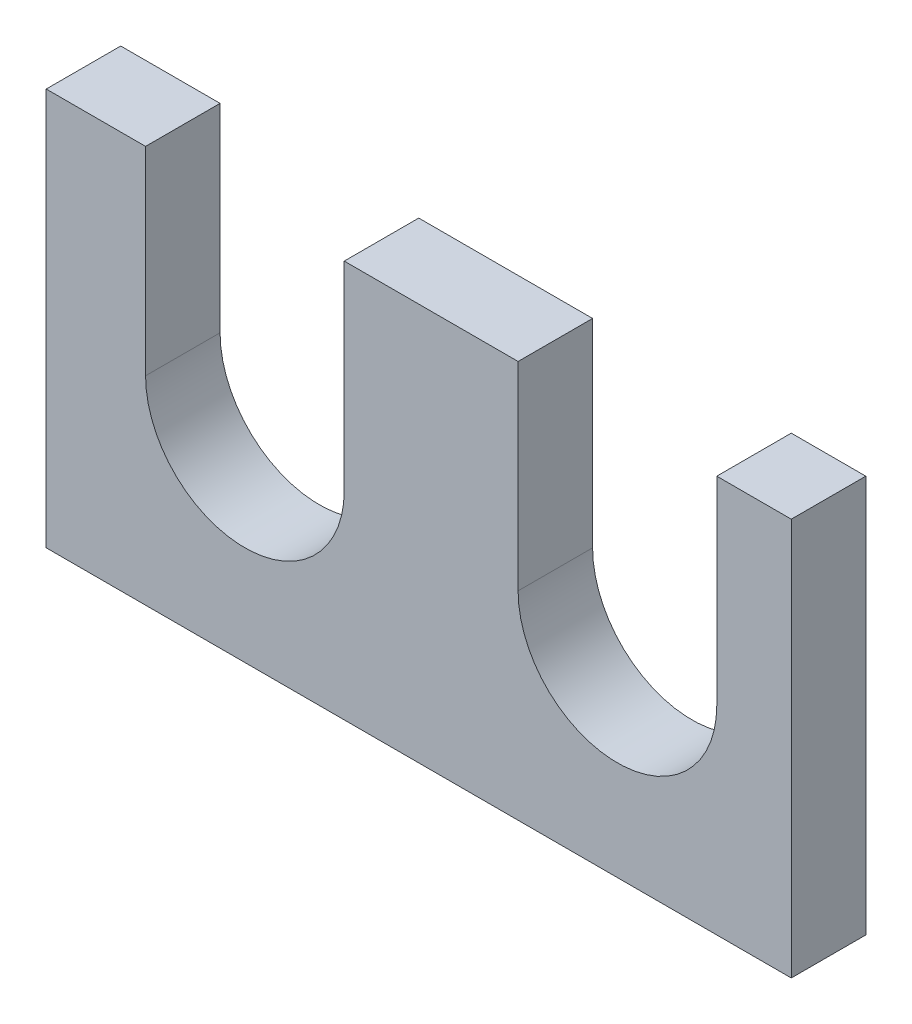
from build123d import *

# Parameters (mm, degrees)
BOSS_EXTRUDE1_DEPTH = 3


with BuildPart() as part:
    # Sketch1 → Boss-Extrude1 (new body)
    with BuildSketch(Plane.XY):
        with BuildLine():
            Line((0, 0), (30, 0))
            Line((30, 0), (30, 16))
            Line((30, 16), (27, 16))
            Line((27, 16), (27, 8))
            ThreePointArc((27, 8), (23, 4), (19, 8))
            Line((19, 8), (19, 16))
            Line((19, 16), (12, 16))
            Line((12, 16), (12, 8))
            ThreePointArc((12, 8), (8, 4), (4, 8))
            Line((4, 8), (4, 16))
            Line((4, 16), (0, 16))
            Line((0, 16), (0, 0))
        make_face()
    extrude(amount=BOSS_EXTRUDE1_DEPTH)


solid = part.part
